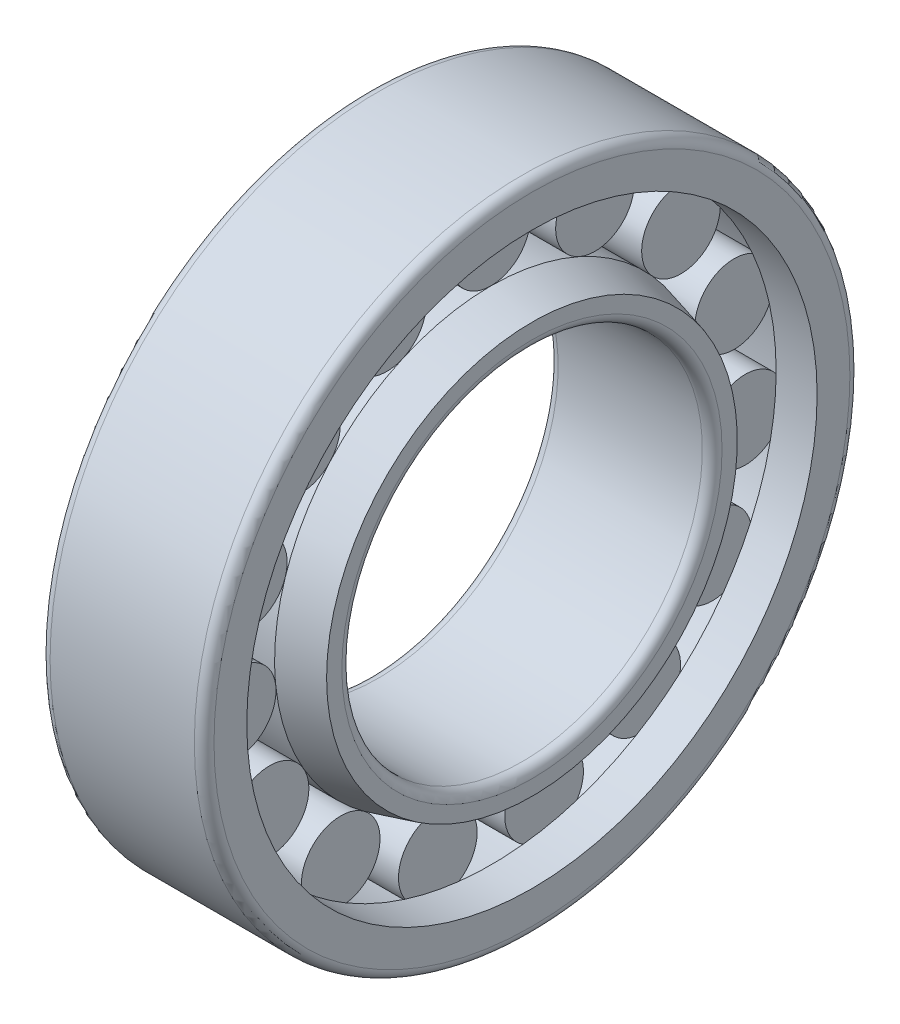
from build123d import *

# Parameters (mm, degrees)
SKETCH3_W         = 12.5
SKETCH3_H         = 6.0001
CIRPATTERN1_COUNT = 15


with BuildPart() as part:
    # Sketch2 → Base-Revolve (revolve)
    with BuildSketch(Plane.XY, mode=Mode.PRIVATE) as base_revolve_sk:
        with BuildLine():
            Line((6.25, 33), (18.75, 33))
            Line((18.75, 33), (25, 31.325317547))
            Line((25, 31.325317547), (25, 29))
            ThreePointArc((25, 29), (24.560660172, 27.939339828), (23.5, 27.5))
            Line((23.5, 27.5), (1.5, 27.5))
            ThreePointArc((1.5, 27.5), (0.439339828, 27.939339828), (0, 29))
            Line((0, 29), (0, 29.47830599))
            Line((0, 29.47830599), (6.25, 33))
        make_face()
    revolve(base_revolve_sk.sketch.rotate(Axis((-10.080094127, 0, 0), (1, 0, 0)), 90), axis=Axis((-10.080094127, 0, 0), (1, 0, 0)))

    # Sketch3 → Boss-Revolve1 (revolve)
    with BuildSketch(Plane.XY):
        with Locations((12.5, 35.99995)):
            Rectangle(SKETCH3_W, SKETCH3_H)
    boss_revolve1 = revolve(axis=Axis((-1.603948851, 39, 0), (1, 0, 0)))

    # Sketch4 → Boss-Revolve2 (revolve)
    with BuildSketch(Plane.XY, mode=Mode.PRIVATE) as boss_revolve2_sk:
        with BuildLine():
            Line((18.75, 43.5), (25, 43.5))
            Line((25, 43.5), (25, 48.5))
            ThreePointArc((25, 48.5), (24.560660172, 49.560660172), (23.5, 50))
            Line((23.5, 50), (1.5, 50))
            ThreePointArc((1.5, 50), (0.439339828, 49.560660172), (0, 48.5))
            Line((0, 48.5), (0, 43.5))
            Line((0, 43.5), (6.25, 43.5))
            Line((6.25, 43.5), (6.25, 45))
            Line((6.25, 45), (18.75, 45))
            Line((18.75, 45), (18.75, 43.5))
        make_face()
    revolve(boss_revolve2_sk.sketch.rotate(Axis((0, 0, 0), (1, 0, 0)), 90), axis=Axis((0, 0, 0), (1, 0, 0)))

    # CirPattern1: Boss-Revolve1 ×15 about axis
    cirpattern1_axis = Axis((0, 0, 0), (1, 0, 0))
    for i in range(1, CIRPATTERN1_COUNT):
        add(boss_revolve1.rotate(cirpattern1_axis, i * 360 / CIRPATTERN1_COUNT))


solid = part.part
